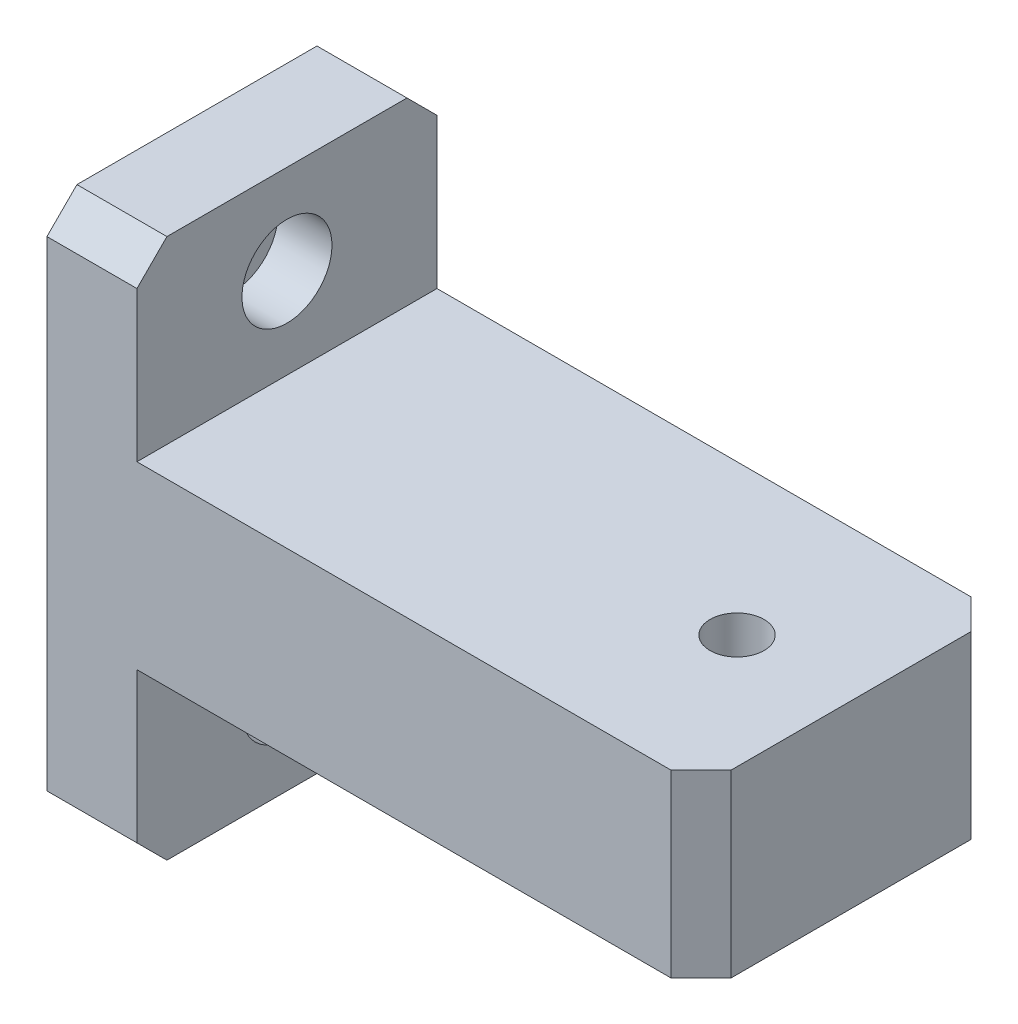
SolidWorks part; units mm, degrees
ref_plane "前视基准面" through (0, 0, 0) normal (0, 0, 1) x (1, 0, 0)
ref_plane "上视基准面" through (0, 0, 0) normal (0, 1, 0) x (1, 0, 0)
ref_plane "右视基准面" through (0, 0, 0) normal (1, 0, 0) x (0, 0, -1)
sketch "草图1" plane through (0, 0, 0) normal (1, 0, 0) x (0, 0, -1)
  line L1 (-50, 15) -> (50, 15)
  line L2 (-50, 15) -> (-50, -15)
  line L3 (-50, -15) -> (50, -15)
  line L4 (50, 15) -> (50, -15)
  line L5 (-50, 15) -> (50, -15) construction
  line L6 (-50, -15) -> (50, 15) construction
  point P0 (0, 0)
  dimension "D1" = 30
  dimension "D2" = 100
extrude "凸台-拉伸1" add sketch "草图1" along normal blind 14
sketch "草图2" plane through (14, 0, 0) normal (1, 0, 0) x (0, 0, -1)
  line L0 (-50, -15) -> (50, -15) construction
  line L1 (-25, 15) -> (25, 15)
  line L2 (-25, 15) -> (-25, -15)
  line L3 (-25, -15) -> (25, -15)
  line L4 (25, 15) -> (25, -15)
  line L5 (-25, 15) -> (25, -15) construction
  line L6 (-25, -15) -> (25, 15) construction
  point P0 (0, 0)
  dimension "D1" = 50
extrude "凸台-拉伸2" add sketch "草图2" along normal blind 95
sketch "草图3" plane through (0, -15, 0) normal (0, -1, 0) x (1, 0, 0)
  circle A0 centre (90, 0) radius 12.5
  dimension "D2" = 25
  dimension "D1" = 90
extrude "切除-拉伸1" cut sketch "草图3" against normal blind 5
hole_wizard "Ø9.0 (9) 直径孔1" positions "草图4" profile "草图5" hole size "Ø9.0" standard "ISO" end condition through all
sketch "草图4" plane through (0, -15, 0) normal (0, -1, 0) x (-1, 0, 0)
  point P0 (-90, 0)
sketch "草图5" plane through (90, -15, 0) normal (1, 0, 0) x (0, 0, -1)
  line L0 (0, 0) -> (0, 30)
  line L1 (0, 30) -> (4.5, 30)
  line L2 (4.5, 30) -> (4.5, 0)
  line L5 (4.5, 0) -> (0, 0)
  line L11 (0, -6.35) -> (0, 107.95) construction
  dimension "通孔孔直径" = 9
  dimension "通孔孔深度" = 30
hole_wizard "Ø9.0 (9) 直径孔2" positions "草图6" profile "草图7" hole size "Ø9.0" standard "ISO" end condition through all
sketch "草图6" plane through (14, 0, 0) normal (1, 0, 0) x (0, 0, -1)
  line L1 (0, 0) -> (0, 40.5166) construction
  point P0 (-40, 0)
  point P2 (40, 0)
  dimension "D1" = 80
sketch "草图7" plane through (14, 0, 40) normal (0, 1, 0) x (0, 0, -1)
  line L0 (0, 0) -> (0, 14)
  line L1 (0, 14) -> (4.5, 14)
  line L2 (4.5, 14) -> (4.5, 0)
  line L5 (4.5, 0) -> (0, 0)
  line L11 (0, -6.35) -> (0, 107.95) construction
  dimension "通孔孔直径" = 9
  dimension "通孔孔深度" = 14
sketch "草图8" plane through (109, 0, 0) normal (1, 0, 0) x (0, 0, -1)
  line L1 (-25, 15) -> (25, 15)
  line L2 (-25, 15) -> (-25, -15)
  line L3 (-25, -15) -> (25, -15)
  line L4 (25, 15) -> (25, -15)
  line L5 (-25, 15) -> (25, -15) construction
  line L6 (-25, -15) -> (25, 15) construction
  point P0 (0, 0)
extrude "切除-拉伸2" cut sketch "草图8" against normal through all flip side to cut
sketch "草图9" plane through (0, -15, 0) normal (0, -1, 0) x (1, 0, 0)
  line L0 (109, -25) -> (0, -25) construction
  line L1 (0, 25) -> (15, 25)
  line L2 (0, 25) -> (0, -25)
  line L3 (0, -25) -> (15, -25)
  line L4 (15, 25) -> (15, -25)
  dimension "D1" = 15
extrude "凸台-拉伸3" add sketch "草图9" along normal blind 30
sketch "草图10" plane through (0, 15, 0) normal (0, 1, 0) x (1, 0, 0)
  line L1 (0, 25) -> (15, 25)
  line L2 (0, 25) -> (0, -25)
  line L3 (0, -25) -> (15, -25)
  line L4 (15, 25) -> (15, -25)
extrude "凸台-拉伸4" add sketch "草图10" along normal blind 30
hole_wizard "打孔尺寸(%根据)内六角圆柱头螺钉的类型1" positions "草图11" profile "草图12" counterbore size "M8" standard "GB" end condition through all
sketch "草图11" plane through (15, 0, 0) normal (1, 0, 0) x (0, 0, -1)
  line L0 (0, 0) -> (0, 61.9295) construction
  line L2 (0, 0) -> (37.5621, 0) construction
  point P0 (0, 30)
  point P2 (0, -30)
  dimension "D1" = 60
sketch "草图12" plane through (15, 30, 0) normal (0, 1, 0) x (0, 0, -1)
  line L0 (0, 0) -> (0, 15)
  line L1 (0, 15) -> (4.5, 15)
  line L3 (4.5, 15) -> (4.5, 9)
  line L4 (4.5, 9) -> (7.5, 9)
  line L5 (7.5, 9) -> (7.5, 0)
  line L7 (7.5, 0) -> (0, 0)
  line L11 (0, -6.35) -> (0, 107.95) construction
  dimension "通孔孔直径" = 9
  dimension "通孔孔深度" = 15
  dimension "柱形沉头孔直径" = 15
  dimension "柱形沉头孔深度" = 9
chamfer "倒角1" distance 5 angle 45 6 edges at (7.5, 45, 25) (7.5, 45, -25) (7.5, -45, 25) (7.5, -45, -25) (109, 0, -25) (109, 0, 25)
